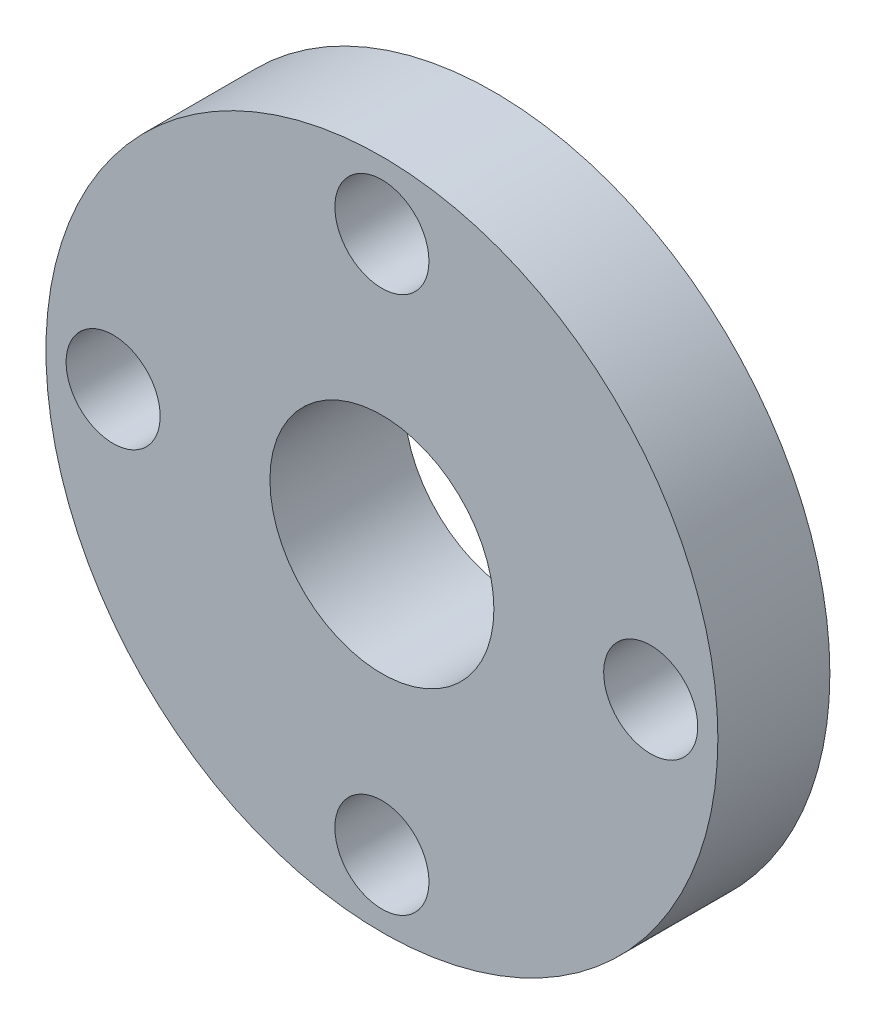
from build123d import *

# Parameters (mm, degrees)
SKETCH1_R           = 15
BOSS_EXTRUDE1_DEPTH = 5
SKETCH2_R           = 2.1
CUT_EXTRUDE1_DEPTH  = 22.794494718
CIRPATTERN1_COUNT   = 4
SKETCH3_R           = 8
BOSS_EXTRUDE2_DEPTH = 1
SKETCH4_R           = 5
CUT_EXTRUDE3_DEPTH  = 23.045407685


with BuildPart() as part:
    # Sketch1 → Boss-Extrude1 (new body)
    with BuildSketch(Plane.XY):
        Circle(SKETCH1_R)
    extrude(amount=BOSS_EXTRUDE1_DEPTH)

    # Sketch2 → Cut-Extrude1 (cut, through all)
    with BuildSketch(Plane.XY.offset(5)):
        with Locations((0, 12)):
            Circle(SKETCH2_R)
    cut_extrude1 = extrude(amount=-CUT_EXTRUDE1_DEPTH, mode=Mode.SUBTRACT)

    # CirPattern1: Cut-Extrude1 ×4 about axis
    cirpattern1_axis = Axis((0, 0, 0), (0, 0, 1))
    for i in range(1, CIRPATTERN1_COUNT):
        add(cut_extrude1.rotate(cirpattern1_axis, i * 360 / CIRPATTERN1_COUNT), mode=Mode.SUBTRACT)

    # Sketch3 → Boss-Extrude2 (add)
    with BuildSketch(Plane(origin=(0, 0, 0), x_dir=(-1, 0, 0), z_dir=(0, 0, -1))):
        with Locations(Location((0, 0, 0), (0, 0, 180))):
            Circle(SKETCH3_R)
    extrude(amount=BOSS_EXTRUDE2_DEPTH)

    # Sketch4 → Cut-Extrude3 (cut, through all)
    with BuildSketch(Plane.XY.offset(5)):
        Circle(SKETCH4_R)
    extrude(amount=-CUT_EXTRUDE3_DEPTH, mode=Mode.SUBTRACT)


solid = part.part
